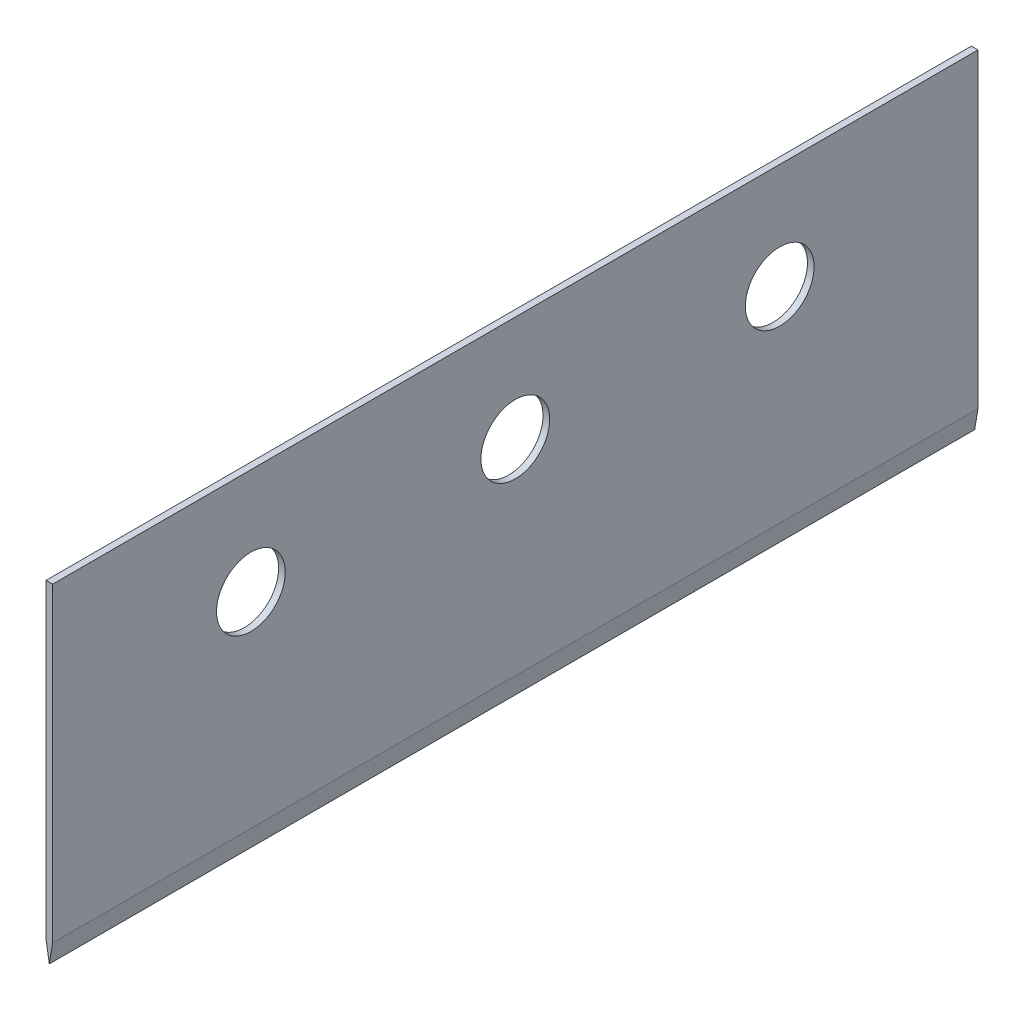
SolidWorks part; units mm, degrees
ref_plane "前视基准面" through (0, 0, 0) normal (0, 0, 1) x (1, 0, 0)
ref_plane "上视基准面" through (0, 0, 0) normal (0, 1, 0) x (1, 0, 0)
ref_plane "右视基准面" through (0, 0, 0) normal (1, 0, 0) x (0, 0, -1)
sketch "草图1" plane through (0, 0, 0) normal (1, 0, 0) x (0, 0, -1)
  line L1 (-35, 12.5) -> (35, 12.5)
  line L2 (-35, 12.5) -> (-35, -12.5)
  line L3 (-35, -12.5) -> (35, -12.5)
  line L4 (35, 12.5) -> (35, -12.5)
  line L5 (-35, 12.5) -> (35, -12.5) construction
  line L6 (-35, -12.5) -> (35, 12.5) construction
  point P0 (0, 0)
  dimension "D1" = 70
  dimension "D2" = 25
extrude "凸台-拉伸1" add sketch "草图1" along normal blind 0.5
sketch "草图2" plane through (0, 0, 35) normal (0, 0, 1) x (1, 0, 0)
  line L0 (0.25, -12.5) -> (0, -11)
  line L1 (0.5, -12.5) -> (0, -12.5) construction
  line L2 (0, 12.5) -> (0, -12.5) construction
  line L3 (0.25, -12.5) -> (0.5, -11)
  line L4 (0.5, 12.5) -> (0.5, -12.5) construction
  line L5 (0, -11) -> (-1.209, -11.2015)
  line L6 (-1.209, -11.2015) -> (-0.5104, -13.1179)
  line L7 (-0.5104, -13.1179) -> (1.3634, -13.1179)
  line L8 (1.3634, -13.1179) -> (1.199, -10.8497)
  line L9 (1.199, -10.8497) -> (0.5, -11)
  dimension "D1" = 1.5
extrude "切除-拉伸1" cut sketch "草图2" against normal through all
hole_wizard "Ø5.2 (5.2) 直径孔1" positions "草图3" profile "草图4" hole size "Ø5.2" standard "GB"
sketch "草图3" plane through (0, 0, 0) normal (-1, 0, 0) x (0, 0, 1)
  line L0 (0, 0) -> (0, 18.8527) construction
  line L2 (-35, 12.5) -> (35, 12.5) construction
  point P0 (-20, 4.5)
  point P2 (0, 4.5)
  point P4 (20, 4.5)
  dimension "D1" = 40
  dimension "D2" = 8
sketch "草图4" plane through (0, 4.5, -20) normal (0, 1, 0) x (0, 0, 1)
  line L0 (0, 0) -> (0, 21.3122)
  line L1 (0, 21.3122) -> (2.6, 19.75)
  line L2 (2.6, 19.75) -> (2.6, 0)
  line L5 (2.6, 0) -> (0, 0)
  line L10 (0, 21.3122) -> (-2.6, 19.75) construction
  line L11 (0, -6.35) -> (0, 107.95) construction
  dimension "孔直径" = 5.2
  dimension "孔深度" = 19.75
  dimension "导头角度" = 118
